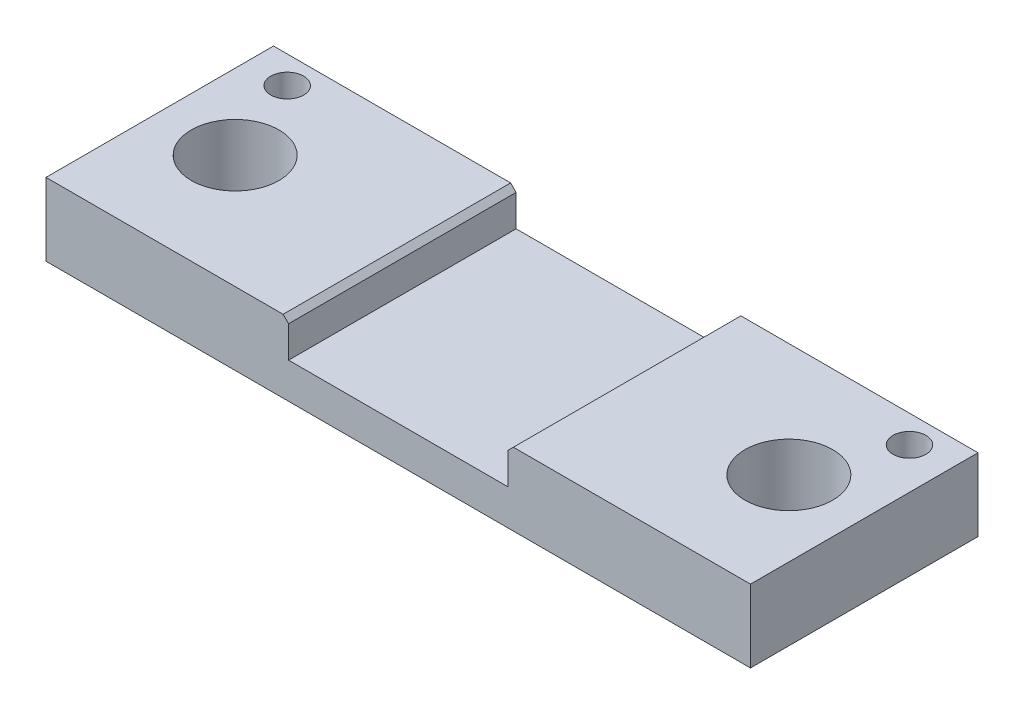
from build123d import *

# Parameters (mm, degrees)
SKETCH1_W           = 25.7
SKETCH1_H           = 8.3
SKETCH1_R           = 1.6
SKETCH1_R_2         = 0.6
BOSS_EXTRUDE1_DEPTH = 2.65
SKETCH2_W           = 8
SKETCH2_H           = 8.3
CUT_EXTRUDE1_DEPTH  = 1.35
CHAMFER1_SIZE       = 0.2


with BuildPart() as part:
    # Sketch1 → Boss-Extrude1 (new body)
    with BuildSketch(Plane(origin=(0, 0, 0), x_dir=(1, 0, 0), z_dir=(0, 1, 0))):
        Rectangle(SKETCH1_W, SKETCH1_H)
        with Locations(Location((-10.1, 0, 0), (0, 0, 270))):
            Circle(SKETCH1_R, mode=Mode.SUBTRACT)
        with Locations(Location((-11.35, 3.15, 0), (0, 0, 270))):
            Circle(SKETCH1_R_2, mode=Mode.SUBTRACT)
        with Locations(Location((11.35, 3.15, 0), (0, 0, 90))):
            Circle(SKETCH1_R_2, mode=Mode.SUBTRACT)
        with Locations(Location((10.1, 0, 0), (0, 0, 90))):
            Circle(SKETCH1_R, mode=Mode.SUBTRACT)
    extrude(amount=BOSS_EXTRUDE1_DEPTH)

    # Sketch2 → Cut-Extrude1 (cut)
    with BuildSketch(Plane(origin=(0, 2.65, 0), x_dir=(1, 0, 0), z_dir=(0, 1, 0))):
        Rectangle(SKETCH2_W, SKETCH2_H)
    extrude(amount=-CUT_EXTRUDE1_DEPTH, mode=Mode.SUBTRACT)

    # Chamfer1
    chamfer1_edges = [part.edges().sort_by_distance(p)[0] for p in [
        (4, 2.65, 0),
        (-4, 2.65, 0),
    ]]
    chamfer(chamfer1_edges, length=CHAMFER1_SIZE)


solid = part.part
